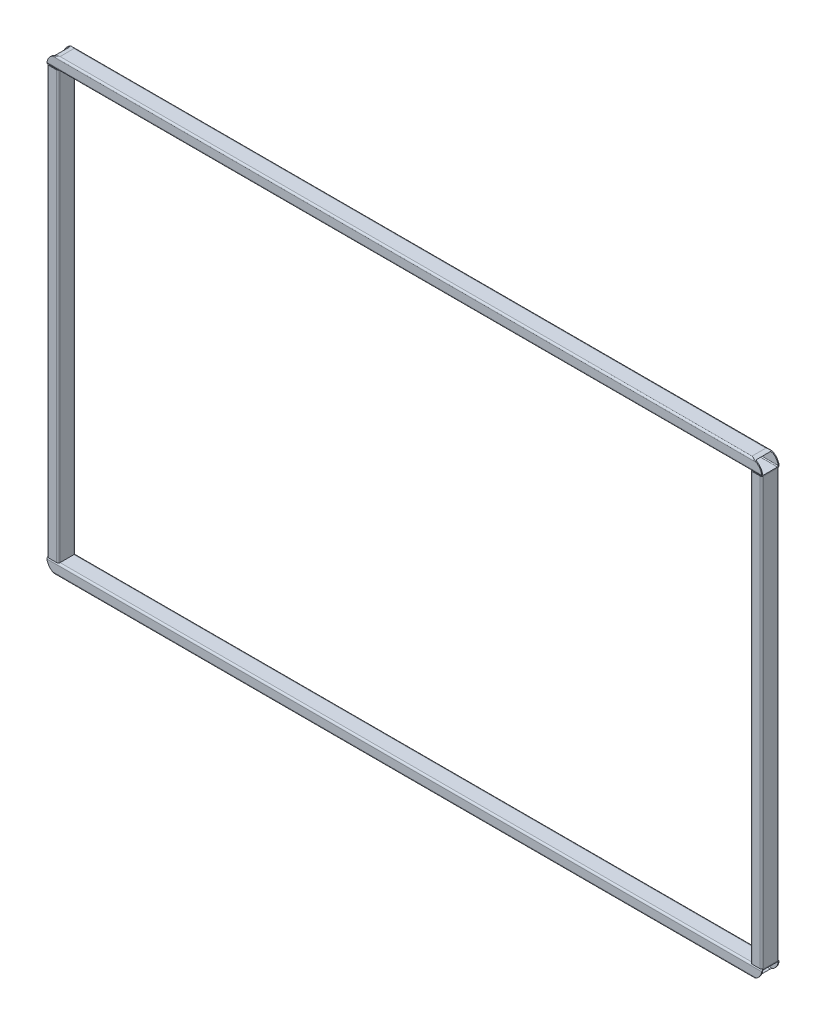
SolidWorks part; units mm, degrees
ref_plane "Front Plane" through (0, 0, 0) normal (0, 0, 1) x (1, 0, 0)
ref_plane "Top Plane" through (0, 0, 0) normal (0, 1, 0) x (1, 0, 0)
ref_plane "Right Plane" through (0, 0, 0) normal (1, 0, 0) x (0, 0, -1)
other "Configuration Table"
sketch3d "3DSketch1"
  line L1 (0, 0, 0) -> (2440, 0, 0)
  line L2 (0, 0, 0) -> (0, 1520, 0)
  line L3 (0, 1520, 0) -> (2440, 1520, 0)
  line L4 (2440, 0, 0) -> (2440, 1520, 0)
  dimension "D1" = 1520
  dimension "D2" = 2440
other "GB/6728-1986 rect hollow section 060 X 40 X 3(1)"
ref_plane "Plane1" through (0, 1520, 0) normal (1, 0, 0) x (0, 1, 0)
sketch "Sketch14" plane through (0, 1520, 0) normal (1, 0, 0) x (0, 1, 0)
  line L0 (-14, -27) -> (14, -27)
  line L1 (-17, -24) -> (-17, 24)
  line L2 (14, 27) -> (-14, 27)
  line L3 (17, 24) -> (17, -24)
  line L4 (-14, -30) -> (14, -30)
  line L5 (-20, -24) -> (-20, 24)
  line L6 (14, 30) -> (-14, 30)
  line L7 (20, 24) -> (20, -24)
  arc A0 (20, 24) -> (14, 30) centre (14, 24) ccw
  arc A1 (14, -30) -> (20, -24) centre (14, -24) ccw
  arc A2 (-20, -24) -> (-14, -30) centre (-14, -24) ccw
  arc A3 (-14, 30) -> (-20, 24) centre (-14, 24) ccw
  arc A4 (-14, 27) -> (-17, 24) centre (-14, 24) ccw
  arc A5 (17, 24) -> (14, 27) centre (14, 24) ccw
  arc A6 (14, -27) -> (17, -24) centre (14, -24) ccw
  arc A7 (-17, -24) -> (-14, -27) centre (-14, -24) ccw
  point P0 (0, 30)
  point P1 (20, 0)
  point P2 (0, -30)
  point P3 (-20, 0)
  point P4 (-20, 30)
  point P5 (20, 30)
  point P6 (20, -30)
  point P7 (-20, -30)
  point P8 (0, 0)
  point P33 (0, 0)
  dimension "D1" = 6
  dimension "Thickness" = 3
  dimension "V_leg" = 60
  dimension "H_leg" = 40
sketch "Sketch2" plane through (0, 1470, 30) normal (0, 0, 1) x (1, 0, 0)
  line L4 (-14, -710) -> (2454, -710) construction
  line L7 (-14, 30) -> (-14, -1450) construction
  line L16 (2454, 30) -> (2454, -1450) construction
  line L17 (1220, 64) -> (1220, -1484) construction
  line L18 (2460, 64) -> (-20, 64) construction
  line L19 (2460, -1484) -> (-20, -1484) construction
  line L20 (2460, -1490) -> (-20, -1490) construction
  line L21 (-20, -1450) -> (-20, -1490)
  line L22 (-20, -1490) -> (20, -1490)
  line L24 (-20, 70) -> (20, 70)
  line L25 (-20, 30) -> (-20, 70)
  line L26 (2460, -1490) -> (2420, -1490)
  line L27 (2460, -1450) -> (2460, -1490)
  line L28 (2460, 30) -> (2460, 70)
  line L29 (2460, 70) -> (2420, 70)
  arc A5 (-20, -1450) -> (20, -1490) centre (20, -1450) ccw
  arc A6 (-20, 30) -> (20, 70) centre (20, 30) cw
  arc A7 (2460, -1450) -> (2420, -1490) centre (2420, -1450) cw
  arc A8 (2460, 30) -> (2420, 70) centre (2420, 30) ccw
  dimension "D1" = 40
extrude "Cut-Extrude1" cut sketch "Sketch2" against normal through all
